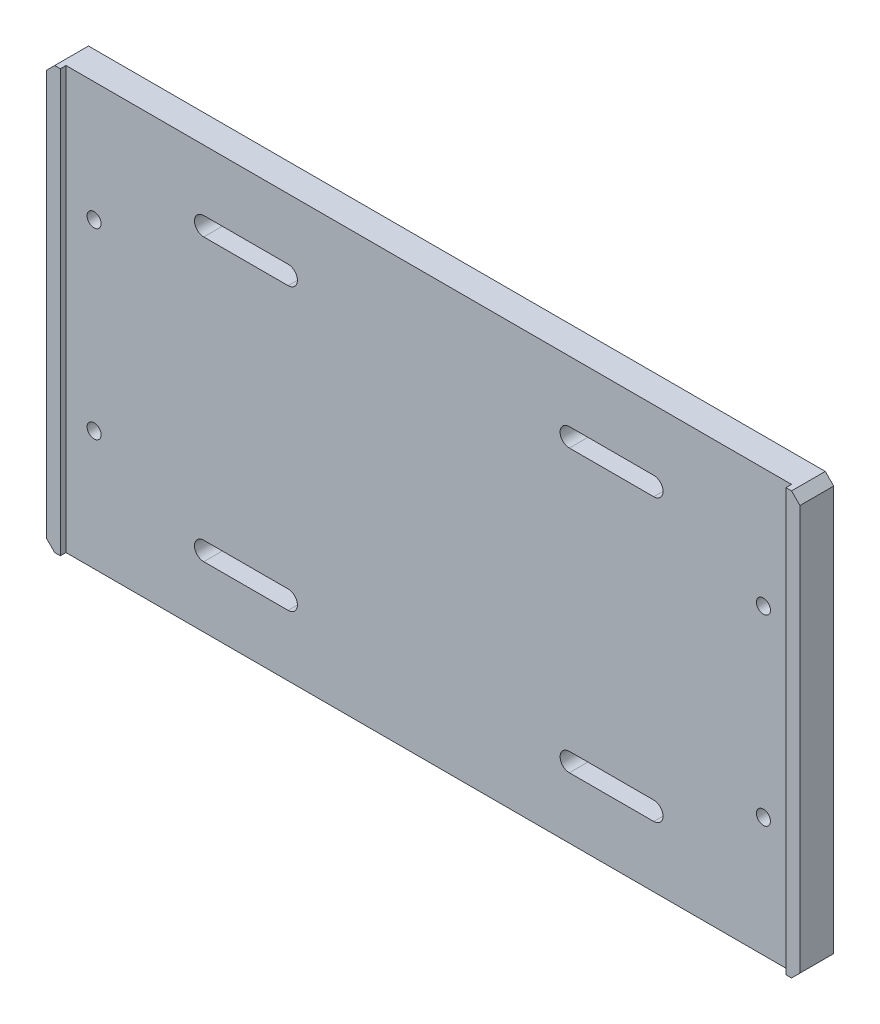
from build123d import *

# Parameters (mm, degrees)
SKETCH_1_W          = 268
SKETCH_1_H          = 150
EXTRUDE_1_DEPTH     = 12
SKETCH_2_W          = 258
SKETCH_2_H          = 150
CUT_EXTRUDE_1_DEPTH = 2
CUT_EXTRUDE_2_DEPTH = 154.886321679
HOLE_WIZARD_M6_1_D  = 5
CHAMFER_1_SIZE      = 3


with BuildPart() as part:
    # 草图1 → 凸台-拉伸1 (new body)
    with BuildSketch(Plane.XY):
        Rectangle(SKETCH_1_W, SKETCH_1_H)
    extrude(amount=EXTRUDE_1_DEPTH)

    # 草图2 → 切除-拉伸1 (cut)
    with BuildSketch(Plane.XY.offset(12)):
        Rectangle(SKETCH_2_W, SKETCH_2_H)
    extrude(amount=-CUT_EXTRUDE_1_DEPTH, mode=Mode.SUBTRACT)

    # 草图3 → 切除-拉伸2 (cut, through all)
    with BuildSketch(Plane.XY.offset(10)):
        with BuildLine():
            Line((-80, 53.3), (-50, 53.3))
            ThreePointArc((-50, 53.3), (-46.7, 50), (-50, 46.7))
            Line((-50, 46.7), (-80, 46.7))
            ThreePointArc((-80, 46.7), (-83.3, 50), (-80, 53.3))
        make_face()
        with BuildLine():
            Line((50, 53.3), (80, 53.3))
            ThreePointArc((80, 53.3), (83.3, 50), (80, 46.7))
            Line((80, 46.7), (50, 46.7))
            ThreePointArc((50, 46.7), (46.7, 50), (50, 53.3))
        make_face()
        with BuildLine():
            Line((-80, -46.7), (-50, -46.7))
            ThreePointArc((-50, -46.7), (-46.7, -50), (-50, -53.3))
            Line((-50, -53.3), (-80, -53.3))
            ThreePointArc((-80, -53.3), (-83.3, -50), (-80, -46.7))
        make_face()
        with BuildLine():
            Line((50, -46.7), (80, -46.7))
            ThreePointArc((80, -46.7), (83.3, -50), (80, -53.3))
            Line((80, -53.3), (50, -53.3))
            ThreePointArc((50, -53.3), (46.7, -50), (50, -46.7))
        make_face()
    extrude(amount=-CUT_EXTRUDE_2_DEPTH, mode=Mode.SUBTRACT)

    # M6 螺纹孔1 (through all)
    with Locations(Plane.XY.offset(10)):
        with Locations((-119, 32.5), (-119, -32.5), (119, 32.5), (119, -32.5)):
            Hole(HOLE_WIZARD_M6_1_D / 2)

    # 倒角1
    chamfer_1_edges = [part.edges().sort_by_distance(p)[0] for p in [
        (134, -75, 6),
        (-134, -75, 6),
        (-134, 75, 6),
        (134, 75, 6),
    ]]
    chamfer(chamfer_1_edges, length=CHAMFER_1_SIZE)


solid = part.part
